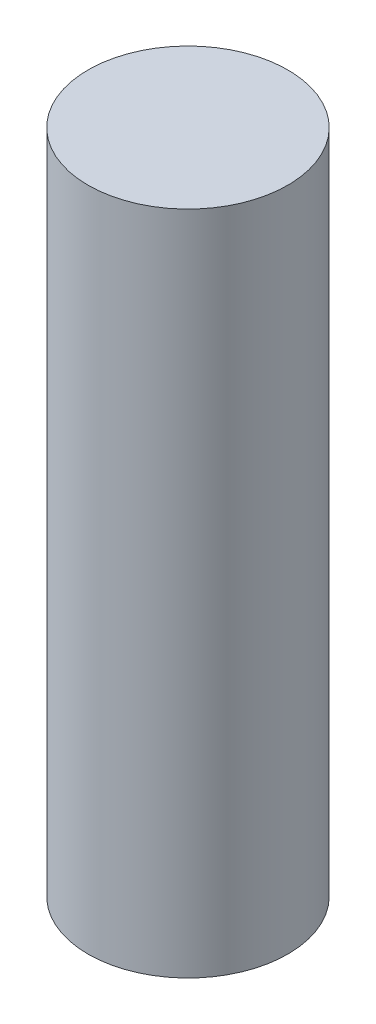
SolidWorks part; units mm, degrees
ref_plane "Front Plane" through (0, 0, 0) normal (0, 0, 1) x (1, 0, 0)
ref_plane "Top Plane" through (0, 0, 0) normal (0, 1, 0) x (1, 0, 0)
ref_plane "Right Plane" through (0, 0, 0) normal (1, 0, 0) x (0, 0, -1)
sketch "Sketch1" plane through (0, 0, 0) normal (0, 1, 0) x (1, 0, 0)
  circle A0 centre (0, 0) radius 15
  dimension "D1" = 30
extrude "Boss-Extrude1" add sketch "Sketch1" along normal mid plane 100
sketch "Sketch2" plane through (0, -50, 0) normal (0, -1, 0) x (1, 0, 0)
  circle A0 centre (0, 0) radius 10
  dimension "D1" = 20
hole_wizard "M20 Tapped Hole1" positions "3DSketch1" profile "Sketch3" tap size "M20" standard "GB"
sketch3d "3DSketch1"
  point P0 (0, -50, 0)
sketch "Sketch3" plane through (0, -50, 0) normal (1, 0, 0) x (0, 0, -1)
  line L0 (0, 0) -> (0, 67.7575)
  line L1 (0, 67.7575) -> (8.75, 62.5)
  line L2 (8.75, 62.5) -> (8.75, 0)
  line L5 (8.75, 0) -> (0, 0)
  line L10 (0, 67.7575) -> (-8.75, 62.5) construction
  line L11 (0, -6.35) -> (0, 107.95) construction
  dimension "螺纹孔钻头直径" = 17.5
  dimension "螺纹孔钻头深度" = 62.5
  dimension "导头角度" = 118
cosmetic thread "Hole Cosmetic Thread1" parameters "D1"=50, "D2"=20
ref_plane "Plane1" through (0, 0, 0) normal (0, -1, 0) x (-1, 0, 0)
